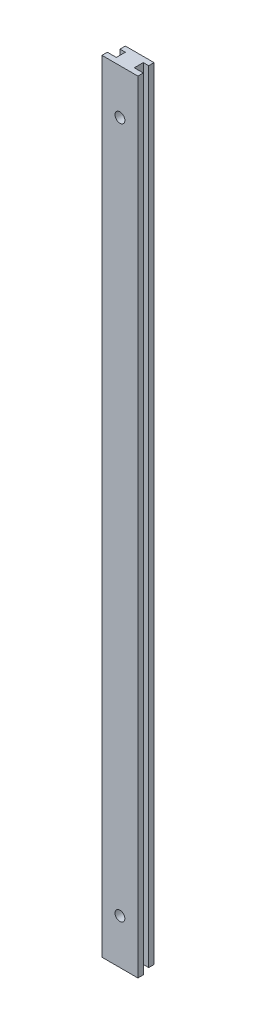
SolidWorks part; units mm, degrees
ref_plane "Front Plane" through (0, 0, 0) normal (0, 0, 1) x (1, 0, 0)
ref_plane "Top Plane" through (0, 0, 0) normal (0, 1, 0) x (1, 0, 0)
ref_plane "Right Plane" through (0, 0, 0) normal (1, 0, 0) x (0, 0, -1)
sketch "Sketch1" plane through (0, 0, 0) normal (0, 1, 0) x (1, 0, 0)
  line L0 (0, 0) -> (20, 0)
  line L1 (20, 0) -> (20, 3)
  line L2 (20, 3) -> (15, 3)
  line L3 (15, 3) -> (15, 8)
  line L4 (18, 8) -> (18, 11)
  line L5 (18, 11) -> (2, 11)
  line L6 (2, 11) -> (2, 8)
  line L7 (2, 8) -> (5, 8)
  line L8 (5, 8) -> (5, 3)
  line L9 (5, 3) -> (0, 3)
  line L10 (0, 3) -> (0, 0)
  line L11 (15, 8) -> (18, 8)
  dimension "D1" = 20
  dimension "D2" = 3
  dimension "D3" = 3
  dimension "D4" = 5
  dimension "D5" = 5
  dimension "D6" = 5
  dimension "D7" = 5
  dimension "D8" = 3
  dimension "D9" = 3
  dimension "D10" = 3
  dimension "D11" = 16
extrude "Boss-Extrude1" add sketch "Sketch1" along normal blind 435
sketch "Sketch2" plane through (0, 0, 0) normal (0, 0, 1) x (1, 0, 0)
  line L0 (0, 435) -> (20, 435) construction
  line L1 (0, 0) -> (20, 0) construction
  line L2 (0, 435) -> (0, 0) construction
  circle A0 centre (10, 410) radius 2.75
  circle A1 centre (10, 25) radius 2.75
  dimension "D1" = 25
  dimension "D2" = 25
  dimension "D3" = 10
  dimension "D5" = 5.5
  dimension "D6" = 5.5
  dimension "D4" = 10
extrude "Cut-Extrude1" cut sketch "Sketch2" against normal blind 5
